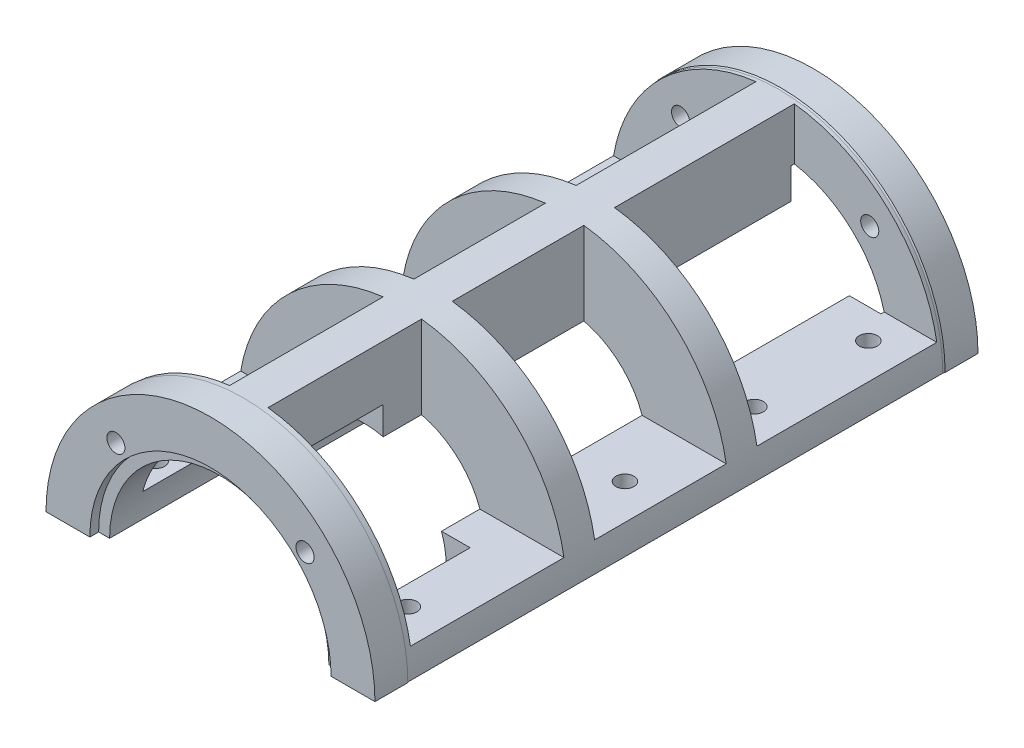
SolidWorks part; units mm, degrees
ref_plane "Front Plane" through (0, 0, 0) normal (0, 0, 1) x (1, 0, 0)
ref_plane "Top Plane" through (0, 0, 0) normal (0, 1, 0) x (1, 0, 0)
ref_plane "Right Plane" through (0, 0, 0) normal (1, 0, 0) x (0, 0, -1)
ref_plane "Plane1" through (0, 234.744, 0) normal (0, -1, 0) x (1, 0, 0)
sketch "Sketch1" plane through (0, 234.744, 0) normal (0, -1, 0) x (1, 0, 0)
  line L0 (371.2306, -1070.693) -> (521.2306, -1070.693)
  line L1 (521.2306, -1070.693) -> (521.2306, -520.693)
  line L2 (521.2306, -520.693) -> (371.2306, -520.693)
  line L3 (371.2306, -520.693) -> (371.2306, -550.693)
  line L4 (371.2306, -550.693) -> (371.7306, -550.693)
  line L5 (371.7306, -550.693) -> (371.7306, -1039.0347)
  line L6 (371.2306, -1040.693) -> (371.2306, -1070.693)
  line L7 (521.2306, -1070.693) -> (521.2306, -520.693) construction
  arc A0 (371.7306, -1039.0347) -> (371.2306, -1040.693) centre (368.7306, -1039.0347) cw
  dimension "D1" = 3
  dimension "D2" = 149.5
  dimension "D3" = 150
  dimension "D4" = 30
  dimension "D6" = 520
  dimension "D7" = 550
revolve "Revolve1" add sketch "Sketch1" angle 180 about L7
ref_plane "Plane2" through (0, 0, -1035.693) normal (0, 0, -1) x (-1, 0, 0)
sketch "Sketch2" plane through (0, 0, -1035.693) normal (0, 0, -1) x (-1, 0, 0)
  line L0 (-503.7306, 383.2162) -> (-503.7306, 259.744)
  line L1 (-503.7306, 259.744) -> (-373.8358, 259.744)
  arc A0 (-373.8358, 259.744) -> (-503.7306, 383.2162) centre (-521.2306, 234.744) ccw
  dimension "D1" = 149.5
  dimension "D2" = 129.8949
  dimension "D3" = 17.5
extrude "Cut-Extrude1" cut sketch "Sketch2" against normal blind 164
ref_plane "Plane3" through (0, 0, -871.693) normal (0, 0, 1) x (1, 0, 0)
sketch "Sketch3" plane through (0, 0, -871.693) normal (0, 0, 1) x (1, 0, 0)
  line L0 (538.7306, 383.2162) -> (538.7306, 259.744)
  line L1 (538.7306, 259.744) -> (668.6255, 259.744)
  arc A0 (668.6255, 259.744) -> (538.7306, 383.2162) centre (521.2306, 234.744) ccw
  dimension "D1" = 149.5
  dimension "D2" = 129.8949
  dimension "D3" = 17.5
extrude "Cut-Extrude2" cut sketch "Sketch3" against normal blind 164
ref_plane "Plane4" through (0, 0, -555.693) normal (0, 0, 1) x (1, 0, 0)
sketch "Sketch4" plane through (0, 0, -555.693) normal (0, 0, 1) x (1, 0, 0)
  line L0 (503.7306, 259.744) -> (503.7306, 383.2162)
  line L1 (373.8358, 259.744) -> (503.7306, 259.744)
  arc A0 (503.7306, 383.2162) -> (373.8358, 259.744) centre (521.2306, 234.744) ccw
  dimension "D1" = 149.5
  dimension "D2" = 17.5
  dimension "D3" = 129.8949
extrude "Cut-Extrude3" cut sketch "Sketch4" against normal blind 140
ref_plane "Plane5" through (0, 0, -843.693) normal (0, 0, -1) x (-1, 0, 0)
sketch "Sketch5" plane through (0, 0, -843.693) normal (0, 0, -1) x (-1, 0, 0)
  line L0 (-503.7306, 259.744) -> (-373.8358, 259.744)
  line L1 (-503.7306, 383.2162) -> (-503.7306, 259.744)
  arc A0 (-373.8358, 259.744) -> (-503.7306, 383.2162) centre (-521.2306, 234.744) ccw
  dimension "D1" = 149.5
  dimension "D2" = 129.8949
  dimension "D3" = 17.5
extrude "Cut-Extrude4" cut sketch "Sketch5" against normal blind 120
sketch "Sketch6" plane through (0, 0, -555.693) normal (0, 0, 1) x (1, 0, 0)
  line L0 (538.7306, 259.744) -> (668.6255, 259.744)
  line L1 (538.7306, 383.2162) -> (538.7306, 259.744)
  arc A0 (668.6255, 259.744) -> (538.7306, 383.2162) centre (521.2306, 234.744) ccw
  dimension "D1" = 149.5
  dimension "D2" = 129.8949
  dimension "D3" = 17.5
extrude "Cut-Extrude5" cut sketch "Sketch6" against normal blind 140
sketch "Sketch7" plane through (0, 0, -843.693) normal (0, 0, -1) x (-1, 0, 0)
  line L0 (-538.7306, 259.744) -> (-538.7306, 383.2162)
  line L1 (-668.6255, 259.744) -> (-538.7306, 259.744)
  arc A0 (-538.7306, 383.2162) -> (-668.6255, 259.744) centre (-521.2306, 234.744) ccw
  dimension "D1" = 149.5
  dimension "D2" = 17.5
  dimension "D3" = 129.8949
extrude "Cut-Extrude6" cut sketch "Sketch7" against normal blind 120
sketch "Sketch8" plane through (0, 234.744, 0) normal (0, -1, 0) x (1, 0, 0)
  line L0 (631.2306, -520.693) -> (521.2306, -520.693)
  line L1 (521.2306, -520.693) -> (521.2306, -1070.693)
  line L2 (521.2306, -1070.693) -> (631.2306, -1070.693)
  line L3 (631.2306, -1070.693) -> (631.2306, -1062.693)
  line L4 (631.2306, -1062.693) -> (623.7306, -1062.693)
  line L5 (623.7306, -1062.693) -> (623.7306, -1032.693)
  line L6 (623.7306, -1032.693) -> (596.2306, -1032.693)
  line L7 (596.2306, -1032.693) -> (596.2306, -660.693)
  line L8 (596.2306, -660.693) -> (621.2306, -660.693)
  line L9 (621.2306, -660.693) -> (621.2306, -528.693)
  line L10 (621.2306, -528.693) -> (631.2306, -528.693)
  line L11 (631.2306, -528.693) -> (631.2306, -520.693)
  line L12 (521.2306, -520.693) -> (521.2306, -1070.693) construction
  dimension "D1" = 75
  dimension "D2" = 100
  dimension "D3" = 102.5
  dimension "D4" = 110
  dimension "D5" = 8
  dimension "D6" = 38
  dimension "D7" = 410
  dimension "D8" = 542
  dimension "D9" = 550
revolve "Cut-Revolve1" cut sketch "Sketch8" angle 360 about L12
sketch "Sketch9" plane through (0, 234.744, 0) normal (0, -1, 0) x (1, 0, 0)
  line L0 (624.4806, -672.693) -> (614.2306, -672.693)
  line L1 (614.2306, -672.693) -> (614.2306, -1022.693)
  line L2 (614.2306, -1022.693) -> (624.4806, -1022.693)
  line L3 (624.4806, -1022.693) -> (624.4806, -672.693)
  line L4 (614.2306, -672.693) -> (614.2306, -1022.693) construction
  dimension "D1" = 10.25
  dimension "D2" = 350
revolve "Cut-Revolve2" cut sketch "Sketch9" angle 360 about L4
sketch "Sketch10" plane through (0, 234.744, 0) normal (0, -1, 0) x (1, 0, 0)
  line L0 (438.4806, -672.693) -> (428.2306, -672.693)
  line L1 (428.2306, -672.693) -> (428.2306, -1022.693)
  line L2 (428.2306, -1022.693) -> (438.4806, -1022.693)
  line L3 (438.4806, -1022.693) -> (438.4806, -672.693)
  line L4 (428.2306, -672.693) -> (428.2306, -1022.693) construction
  dimension "D1" = 10.25
  dimension "D2" = 350
revolve "Cut-Revolve3" cut sketch "Sketch10" angle 360 about L4
hole_wizard "Ø16.5 (16.5) diameter hole1" positions "Sketch12" profile "Sketch11" hole size "Ø16.5" standard "ANSI Metric"
sketch "Sketch12" plane through (0, 259.744, 0) normal (0, 1, 0) x (1, 0, 0)
  point P0 (636.2306, 1005.693)
  point P1 (636.2306, 901.693)
  point P2 (636.2306, 783.693)
  point P3 (636.2306, 585.693)
  point P4 (406.2306, 1005.693)
  point P5 (406.2306, 901.693)
  point P6 (406.2306, 585.693)
  point P7 (406.2306, 783.693)
sketch "Sketch11" plane through (636.2306, 259.744, -1005.693) normal (1, 0, 0) x (0, 0, 1)
  line L0 (0, 0) -> (0, 25)
  line L1 (0, 25) -> (8.25, 25)
  line L2 (8.25, 25) -> (8.25, 0)
  line L5 (8.25, 0) -> (0, 0)
  line L11 (0, -6.35) -> (0, 107.95) construction
  dimension "通孔孔直径" = 16.5
  dimension "通孔孔深度" = 25
hole_wizard "Ø16.5 (16.5) diameter hole2" positions "Sketch14" profile "Sketch13" hole size "Ø16.5" standard "ANSI Metric"
sketch "Sketch14" plane through (0, 0, -1035.693) normal (0, 0, 1) x (1, 0, 0)
  point P0 (607.4977, 321.011)
  point P1 (434.9636, 321.011)
sketch "Sketch13" plane through (607.4977, 321.011, -1035.693) normal (1, 0, 0) x (0, -1, 0)
  line L0 (0, 0) -> (0, 35)
  line L1 (0, 35) -> (8.25, 35)
  line L2 (8.25, 35) -> (8.25, 0)
  line L5 (8.25, 0) -> (0, 0)
  line L11 (0, -6.35) -> (0, 107.95) construction
  dimension "通孔孔直径" = 16.5
  dimension "通孔孔深度" = 35
hole_wizard "Ø16.5 (16.5) diameter hole3" positions "Sketch16" profile "Sketch15" hole size "Ø16.5" standard "ANSI Metric"
sketch "Sketch16" plane through (0, 0, -555.693) normal (0, 0, -1) x (-1, 0, 0)
  point P0 (-607.4977, 321.011)
  point P1 (-434.9636, 321.011)
sketch "Sketch15" plane through (607.4977, 321.011, -555.693) normal (1, 0, 0) x (0, 1, 0)
  line L0 (0, 0) -> (0, 35)
  line L1 (0, 35) -> (8.25, 35)
  line L2 (8.25, 35) -> (8.25, 0)
  line L5 (8.25, 0) -> (0, 0)
  line L11 (0, -6.35) -> (0, 107.95) construction
  dimension "通孔孔直径" = 16.5
  dimension "通孔孔深度" = 35
